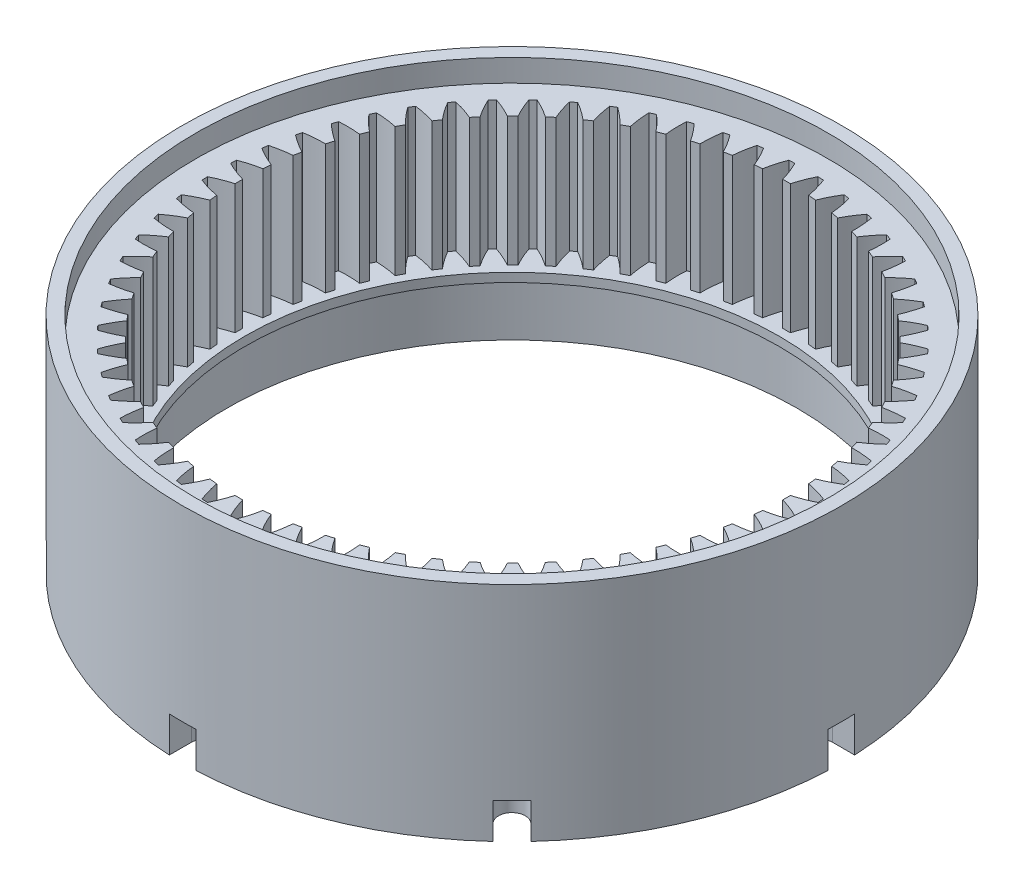
from build123d import *

# Parameters (mm, degrees)
SKETCH1_R           = 37
BOSS_EXTRUDE1_DEPTH = 25
SKETCH2_R           = 35.5
CUT_EXTRUDE1_DEPTH  = 2.5
CUT_EXTRUDE2_DEPTH  = 14.5
SKETCH4_R           = 30
CUT_EXTRUDE3_DEPTH  = 62.5
SKETCH5_R           = 32
CUT_EXTRUDE4_DEPTH  = 7
CUT_EXTRUDE5_DEPTH  = 6
CUT_EXTRUDE6_DEPTH  = 4
CIRPATTERN1_COUNT   = 8


with BuildPart() as part:
    # Sketch1 → Boss-Extrude1 (new body)
    with BuildSketch(Plane(origin=(0, 0, 0), x_dir=(1, 0, 0), z_dir=(0, 1, 0))):
        with Locations(Location((0, 0, 0), (0, 0, 270))):
            Circle(SKETCH1_R)
    extrude(amount=BOSS_EXTRUDE1_DEPTH)

    # Sketch2 → Cut-Extrude1 (cut)
    with BuildSketch(Plane(origin=(0, 25, 0), x_dir=(1, 0, 0), z_dir=(0, 1, 0))):
        with Locations(Location((0, 0, 0), (0, 0, 270))):
            Circle(SKETCH2_R)
    extrude(amount=-CUT_EXTRUDE1_DEPTH, mode=Mode.SUBTRACT)

    # Sketch3 → Cut-Extrude2 (cut)
    with BuildSketch(Plane(origin=(0, 22.5, 0), x_dir=(1, 0, 0), z_dir=(0, 1, 0))):
        with BuildLine():
            ThreePointArc((-33.098118466, 1.500835334), (-32.004134305, 1.015094225), (-30.869559771, 0.633667435))
            ThreePointArc((-30.869559771, 0.633667435), (-30.872535482, 0.205892471), (-30.869559771, -0.221882494))
            ThreePointArc((-30.869559771, -0.221882494), (-32.004134305, -0.603309284), (-33.098118466, -1.089050393))
            ThreePointArc((-33.098118466, -1.089050393), (-33.083785537, -1.413340782), (-33.066263433, -1.737474497))
            ThreePointArc((-33.066263433, -1.737474497), (-31.92993615, -2.113647431), (-30.763438539, -2.382029796))
            ThreePointArc((-30.763438539, -2.382029796), (-30.724470643, -2.808036577), (-30.679579982, -3.233460018))
            ThreePointArc((-30.679579982, -3.233460018), (-31.771304866, -3.724257885), (-32.81241024, -4.314889217))
            ThreePointArc((-32.81241024, -4.314889217), (-32.766360311, -4.636213187), (-32.717151921, -4.957068642))
            ThreePointArc((-32.717151921, -4.957068642), (-31.549424969, -5.22005065), (-30.362238291, -5.37280392))
            ThreePointArc((-30.362238291, -5.37280392), (-30.281702069, -5.792939841), (-30.19532878, -6.211914697))
            ThreePointArc((-30.19532878, -6.211914697), (-31.233690107, -6.80735699), (-32.21189028, -7.497190442))
            ThreePointArc((-32.21189028, -7.497190442), (-32.134566838, -7.812453466), (-32.054146065, -8.12694065))
            ThreePointArc((-32.054146065, -8.12694065), (-30.866265294, -8.274199071), (-29.669822805, -8.309852149))
            ThreePointArc((-29.669822805, -8.309852149), (-29.548493866, -8.72007107), (-29.42146977, -9.128562385))
            ThreePointArc((-29.42146977, -9.128562385), (-30.396467553, -9.822914668), (-31.302341922, -10.605306768))
            ThreePointArc((-31.302341922, -10.605306768), (-31.194489633, -10.911472691), (-31.083630974, -11.216562919))
            ThreePointArc((-31.083630974, -11.216562919), (-29.887036324, -11.246679574), (-28.692860421, -11.164889102))
            ThreePointArc((-28.692860421, -11.164889102), (-28.531907227, -11.561240391), (-28.365455637, -11.95531417))
            ThreePointArc((-28.365455637, -11.95531417), (-29.267700114, -12.741889452), (-30.092524615, -13.609305334))
            ThreePointArc((-30.092524615, -13.609305334), (-29.955182155, -13.903425613), (-29.814953239, -14.196180699))
            ThreePointArc((-29.814953239, -14.196180699), (-28.621168571, -14.108865548), (-27.440759819, -13.910419212))
            ThreePointArc((-27.440759819, -13.910419212), (-27.24173244, -14.28908579), (-27.037456375, -14.664946887))
            ThreePointArc((-27.037456375, -14.664946887), (-27.858258438, -15.536170017), (-28.594089559, -16.480255994))
            ThreePointArc((-28.594089559, -16.480255994), (-28.428579612, -16.759498088), (-28.260330921, -17.037098641))
            ThreePointArc((-28.260330921, -17.037098641), (-27.080853033, -16.833192577), (-25.925579414, -16.520001524))
            ThreePointArc((-25.925579414, -16.520001524), (-25.690394591, -16.877336625), (-25.450261341, -17.231365292))
            ThreePointArc((-25.450261341, -17.231365292), (-26.181716218, -18.178845916), (-26.821467503, -19.190509923))
            ThreePointArc((-26.821467503, -19.190509923), (-26.629384021, -19.452184578), (-26.434735881, -19.711957152))
            ThreePointArc((-26.434735881, -19.711957152), (-25.280923791, -19.393423903), (-24.161911222, -18.968504334))
            ThreePointArc((-24.161911222, -18.968504334), (-23.892833913, -19.301066624), (-23.619156093, -19.629853372))
            ThreePointArc((-23.619156093, -19.629853372), (-24.254219473, -20.644466733), (-24.791729768, -21.713965893))
            ThreePointArc((-24.791729768, -21.713965893), (-24.574922619, -21.955553039), (-24.355749598, -22.194995884))
            ThreePointArc((-24.355749598, -22.194995884), (-23.238715147, -21.764903097), (-22.16674033, -21.232347221))
            ThreePointArc((-22.16674033, -21.232347221), (-21.866361897, -21.536933944), (-21.561775174, -21.837312377))
            ThreePointArc((-21.561775174, -21.837312377), (-22.09433105, -22.909287194), (-22.524423837, -24.026321645))
            ThreePointArc((-22.524423837, -24.026321645), (-22.284980992, -24.245494666), (-22.043393846, -24.462301815))
            ThreePointArc((-22.043393846, -24.462301815), (-20.973894686, -23.92479152), (-19.959281325, -23.28972814))
            ThreePointArc((-19.959281325, -23.28972814), (-19.630494577, -23.56340596), (-19.297932287, -23.832483269))
            ThreePointArc((-19.297932287, -23.832483269), (-19.722851855, -24.951495838), (-20.041385105, -26.105307928))
            ThreePointArc((-20.041385105, -26.105307928), (-19.781612531, -26.299956068), (-19.519937876, -26.492039551))
            ThreePointArc((-19.519937876, -26.492039551), (-18.508273869, -25.852288265), (-17.560793245, -25.120833388))
            ThreePointArc((-17.560793245, -25.120833388), (-17.206764577, -25.360966638), (-16.849429477, -25.596151462))
            ThreePointArc((-16.849429477, -25.596151462), (-17.16262053, -26.75142508), (-17.366526593, -27.930902968))
            ThreePointArc((-17.366526593, -27.930902968), (-17.088926041, -28.09915166), (-16.809683947, -28.264661606))
            ThreePointArc((-16.809683947, -28.264661606), (-15.86559797, -27.528830485), (-14.99437484, -26.708028422))
            ThreePointArc((-14.99437484, -26.708028422), (-14.618513743, -26.912304487), (-14.239847165, -27.111331866))
            ThreePointArc((-14.239847165, -27.111331866), (-14.438293501, -28.291740618), (-14.525608651, -29.485525287))
            ThreePointArc((-14.525608651, -29.485525287), (-14.232853566, -29.625754203), (-13.938733287, -29.763096662))
            ThreePointArc((-13.938733287, -29.763096662), (-13.071317405, -28.938272161), (-12.284742123, -28.036027685))
            ThreePointArc((-12.284742123, -28.036027685), (-11.890668344, -28.202479275), (-11.494317055, -28.363432468))
            ThreePointArc((-11.494317055, -28.363432468), (-11.576107527, -29.557608371), (-11.545990872, -30.754203022))
            ThreePointArc((-11.545990872, -30.754203022), (-11.240900644, -30.865061681), (-10.93473472, -30.97291397))
            ThreePointArc((-10.93473472, -30.97291397), (-10.152342621, -30.0670396), (-9.457990338, -29.092041818))
            ThreePointArc((-9.457990338, -29.092041818), (-9.049499023, -29.219065913), (-8.639280102, -29.340394852))
            ThreePointArc((-8.639280102, -29.340394852), (-8.603627023, -30.536837341), (-8.456368602, -31.724718112))
            ThreePointArc((-8.456368602, -31.724718112), (-8.141881419, -31.805138885), (-7.826618395, -31.882462327))
            ThreePointArc((-7.826618395, -31.882462327), (-7.136784943, -30.904262155), (-6.54134265, -29.865900828))
            ThreePointArc((-6.54134265, -29.865900828), (-6.122367794, -29.952274117), (-5.702231873, -30.032810339))
            ThreePointArc((-5.702231873, -30.032810339), (-5.549478603, -31.219997017), (-5.286496595, -32.387723968))
            ThreePointArc((-5.286496595, -32.387723968), (-4.965641139, -32.436932358), (-4.64431717, -32.482982287))
            ThreePointArc((-4.64431717, -32.482982287), (-4.053685838, -31.441876913), (-3.562887971, -30.350152029))
            ThreePointArc((-3.562887971, -30.350152029), (-3.13746453, -30.39504269), (-2.711457749, -30.434010587))
            ThreePointArc((-2.711457749, -30.434010587), (-2.443075384, -31.600508197), (-2.06690245, -32.73683548))
            ThreePointArc((-2.06690245, -32.73683548), (-1.742768735, -32.754357584), (-1.418478346, -32.768690514))
            ThreePointArc((-1.418478346, -32.768690514), (-0.932737237, -31.674706353), (-0.551310447, -30.540131818))
            ThreePointArc((-0.551310447, -30.540131818), (-0.123535482, -30.543107529), (0.304239482, -30.540131818))
            ThreePointArc((0.304239482, -30.540131818), (0.685666273, -31.674706353), (1.171407382, -32.768690514))
            ThreePointArc((1.171407382, -32.768690514), (1.495697771, -32.754357584), (1.819831485, -32.73683548))
            ThreePointArc((1.819831485, -32.73683548), (2.196004419, -31.600508197), (2.464386784, -30.434010587))
            ThreePointArc((2.464386784, -30.434010587), (2.890393566, -30.39504269), (3.315817006, -30.350152029))
            ThreePointArc((3.315817006, -30.350152029), (3.806614874, -31.441876913), (4.397246205, -32.482982287))
            ThreePointArc((4.397246205, -32.482982287), (4.718570175, -32.436932358), (5.039425631, -32.387723968))
            ThreePointArc((5.039425631, -32.387723968), (5.302407638, -31.219997017), (5.455160909, -30.032810339))
            ThreePointArc((5.455160909, -30.032810339), (5.875296829, -29.952274117), (6.294271685, -29.865900828))
            ThreePointArc((6.294271685, -29.865900828), (6.889713978, -30.904262155), (7.57954743, -31.882462327))
            ThreePointArc((7.57954743, -31.882462327), (7.894810455, -31.805138885), (8.209297638, -31.724718112))
            ThreePointArc((8.209297638, -31.724718112), (8.356556059, -30.536837341), (8.392209137, -29.340394852))
            ThreePointArc((8.392209137, -29.340394852), (8.802428059, -29.219065913), (9.210919373, -29.092041818))
            ThreePointArc((9.210919373, -29.092041818), (9.905271657, -30.0670396), (10.687663756, -30.97291397))
            ThreePointArc((10.687663756, -30.97291397), (10.99382968, -30.865061681), (11.298919907, -30.754203022))
            ThreePointArc((11.298919907, -30.754203022), (11.329036562, -29.557608371), (11.24724609, -28.363432468))
            ThreePointArc((11.24724609, -28.363432468), (11.643597379, -28.202479275), (12.037671158, -28.036027685))
            ThreePointArc((12.037671158, -28.036027685), (12.82424644, -28.938272161), (13.691662323, -29.763096662))
            ThreePointArc((13.691662323, -29.763096662), (13.985782601, -29.625754203), (14.278537687, -29.485525287))
            ThreePointArc((14.278537687, -29.485525287), (14.191222536, -28.291740618), (13.992776201, -27.111331866))
            ThreePointArc((13.992776201, -27.111331866), (14.371442778, -26.912304487), (14.747303875, -26.708028422))
            ThreePointArc((14.747303875, -26.708028422), (15.618527006, -27.528830485), (16.562612982, -28.264661606))
            ThreePointArc((16.562612982, -28.264661606), (16.841855076, -28.09915166), (17.119455629, -27.930902968))
            ThreePointArc((17.119455629, -27.930902968), (16.915549565, -26.75142508), (16.602358513, -25.596151462))
            ThreePointArc((16.602358513, -25.596151462), (16.959693613, -25.360966638), (17.31372228, -25.120833388))
            ThreePointArc((17.31372228, -25.120833388), (18.261202904, -25.852288265), (19.272866911, -26.492039551))
            ThreePointArc((19.272866911, -26.492039551), (19.534541566, -26.299956068), (19.794314141, -26.105307928))
            ThreePointArc((19.794314141, -26.105307928), (19.475780891, -24.951495838), (19.050861322, -23.832483269))
            ThreePointArc((19.050861322, -23.832483269), (19.383423612, -23.56340596), (19.71221036, -23.28972814))
            ThreePointArc((19.71221036, -23.28972814), (20.726823722, -23.92479152), (21.796322881, -24.462301815))
            ThreePointArc((21.796322881, -24.462301815), (22.037910028, -24.245494666), (22.277352872, -24.026321645))
            ThreePointArc((22.277352872, -24.026321645), (21.847260086, -22.909287194), (21.314704209, -21.837312377))
            ThreePointArc((21.314704209, -21.837312377), (21.619290932, -21.536933944), (21.919669365, -21.232347221))
            ThreePointArc((21.919669365, -21.232347221), (22.991644182, -21.764903097), (24.108678633, -22.194995884))
            ThreePointArc((24.108678633, -22.194995884), (24.327851654, -21.955553039), (24.544658803, -21.713965893))
            ThreePointArc((24.544658803, -21.713965893), (24.007148509, -20.644466733), (23.372085128, -19.629853372))
            ThreePointArc((23.372085128, -19.629853372), (23.645762948, -19.301066624), (23.914840257, -18.968504334))
            ThreePointArc((23.914840257, -18.968504334), (25.033852826, -19.393423903), (26.187664916, -19.711957152))
            ThreePointArc((26.187664916, -19.711957152), (26.382313057, -19.452184578), (26.574396539, -19.190509923))
            ThreePointArc((26.574396539, -19.190509923), (25.934645254, -18.178845916), (25.203190377, -17.231365292))
            ThreePointArc((25.203190377, -17.231365292), (25.443323626, -16.877336625), (25.67850845, -16.520001524))
            ThreePointArc((25.67850845, -16.520001524), (26.833782069, -16.833192577), (28.013259956, -17.037098641))
            ThreePointArc((28.013259956, -17.037098641), (28.181508648, -16.759498088), (28.347018594, -16.480255994))
            ThreePointArc((28.347018594, -16.480255994), (27.611187473, -15.536170017), (26.79038541, -14.664946887))
            ThreePointArc((26.79038541, -14.664946887), (26.994661475, -14.28908579), (27.193688855, -13.910419212))
            ThreePointArc((27.193688855, -13.910419212), (28.374097607, -14.108865548), (29.567882275, -14.196180699))
            ThreePointArc((29.567882275, -14.196180699), (29.708111191, -13.903425613), (29.84545365, -13.609305334))
            ThreePointArc((29.84545365, -13.609305334), (29.020629149, -12.741889452), (28.118384673, -11.95531417))
            ThreePointArc((28.118384673, -11.95531417), (28.284836263, -11.561240391), (28.445789456, -11.164889102))
            ThreePointArc((28.445789456, -11.164889102), (29.63996536, -11.246679574), (30.83656001, -11.216562919))
            ThreePointArc((30.83656001, -11.216562919), (30.947418669, -10.911472691), (31.055270958, -10.605306768))
            ThreePointArc((31.055270958, -10.605306768), (30.149396589, -9.822914668), (29.174398806, -9.128562385))
            ThreePointArc((29.174398806, -9.128562385), (29.301422901, -8.72007107), (29.422751841, -8.309852149))
            ThreePointArc((29.422751841, -8.309852149), (30.619194329, -8.274199071), (31.807075101, -8.12694065))
            ThreePointArc((31.807075101, -8.12694065), (31.887495873, -7.812453466), (31.964819316, -7.497190442))
            ThreePointArc((31.964819316, -7.497190442), (30.986619143, -6.80735699), (29.948257816, -6.211914697))
            ThreePointArc((29.948257816, -6.211914697), (30.034631105, -5.792939841), (30.115167327, -5.37280392))
            ThreePointArc((30.115167327, -5.37280392), (31.302354005, -5.22005065), (32.470080956, -4.957068642))
            ThreePointArc((32.470080956, -4.957068642), (32.519289347, -4.636213187), (32.565339276, -4.314889217))
            ThreePointArc((32.565339276, -4.314889217), (31.524233902, -3.724257885), (30.432509017, -3.233460018))
            ThreePointArc((30.432509017, -3.233460018), (30.477399678, -2.808036577), (30.516367575, -2.382029796))
            ThreePointArc((30.516367575, -2.382029796), (31.682865186, -2.113647431), (32.819192468, -1.737474497))
            ThreePointArc((32.819192468, -1.737474497), (32.836714572, -1.413340782), (32.851047502, -1.089050393))
            ThreePointArc((32.851047502, -1.089050393), (31.757063341, -0.603309284), (30.622488807, -0.221882494))
            ThreePointArc((30.622488807, -0.221882494), (30.625464518, 0.205892471), (30.622488807, 0.633667435))
            ThreePointArc((30.622488807, 0.633667435), (31.757063341, 1.015094225), (32.851047502, 1.500835334))
            ThreePointArc((32.851047502, 1.500835334), (32.836714572, 1.825125723), (32.819192468, 2.149259438))
            ThreePointArc((32.819192468, 2.149259438), (31.682865186, 2.525432372), (30.516367575, 2.793814737))
            ThreePointArc((30.516367575, 2.793814737), (30.477399678, 3.219821519), (30.432509017, 3.645244959))
            ThreePointArc((30.432509017, 3.645244959), (31.524233902, 4.136042826), (32.565339276, 4.726674158))
            ThreePointArc((32.565339276, 4.726674158), (32.519289347, 5.047998128), (32.470080956, 5.368853583))
            ThreePointArc((32.470080956, 5.368853583), (31.302354005, 5.631835591), (30.115167327, 5.784588861))
            ThreePointArc((30.115167327, 5.784588861), (30.034631105, 6.204724782), (29.948257816, 6.623699638))
            ThreePointArc((29.948257816, 6.623699638), (30.986619143, 7.219141931), (31.964819316, 7.908975383))
            ThreePointArc((31.964819316, 7.908975383), (31.887495873, 8.224238407), (31.807075101, 8.538725591))
            ThreePointArc((31.807075101, 8.538725591), (30.619194329, 8.685984012), (29.422751841, 8.72163709))
            ThreePointArc((29.422751841, 8.72163709), (29.301422901, 9.131856011), (29.174398806, 9.540347326))
            ThreePointArc((29.174398806, 9.540347326), (30.149396589, 10.234699609), (31.055270958, 11.017091709))
            ThreePointArc((31.055270958, 11.017091709), (30.947418669, 11.323257632), (30.83656001, 11.62834786))
            ThreePointArc((30.83656001, 11.62834786), (29.63996536, 11.658464515), (28.445789456, 11.576674043))
            ThreePointArc((28.445789456, 11.576674043), (28.284836263, 11.973025332), (28.118384673, 12.367099111))
            ThreePointArc((28.118384673, 12.367099111), (29.020629149, 13.153674393), (29.84545365, 14.021090275))
            ThreePointArc((29.84545365, 14.021090275), (29.708111191, 14.315210554), (29.567882275, 14.60796564))
            ThreePointArc((29.567882275, 14.60796564), (28.374097607, 14.520650489), (27.193688855, 14.322204153))
            ThreePointArc((27.193688855, 14.322204153), (26.994661475, 14.700870731), (26.79038541, 15.076731828))
            ThreePointArc((26.79038541, 15.076731828), (27.611187473, 15.947954959), (28.347018594, 16.892040935))
            ThreePointArc((28.347018594, 16.892040935), (28.181508648, 17.171283029), (28.013259956, 17.448883582))
            ThreePointArc((28.013259956, 17.448883582), (26.833782069, 17.244977518), (25.67850845, 16.931786465))
            ThreePointArc((25.67850845, 16.931786465), (25.443323626, 17.289121566), (25.203190377, 17.643150233))
            ThreePointArc((25.203190377, 17.643150233), (25.934645254, 18.590630857), (26.574396539, 19.602294864))
            ThreePointArc((26.574396539, 19.602294864), (26.382313057, 19.863969519), (26.187664916, 20.123742093))
            ThreePointArc((26.187664916, 20.123742093), (25.033852826, 19.805208844), (23.914840257, 19.380289275))
            ThreePointArc((23.914840257, 19.380289275), (23.645762948, 19.712851565), (23.372085128, 20.041638313))
            ThreePointArc((23.372085128, 20.041638313), (24.007148509, 21.056251674), (24.544658803, 22.125750834))
            ThreePointArc((24.544658803, 22.125750834), (24.327851654, 22.36733798), (24.108678633, 22.606780825))
            ThreePointArc((24.108678633, 22.606780825), (22.991644182, 22.176688038), (21.919669365, 21.644132162))
            ThreePointArc((21.919669365, 21.644132162), (21.619290932, 21.948718885), (21.314704209, 22.249097318))
            ThreePointArc((21.314704209, 22.249097318), (21.847260086, 23.321072135), (22.277352872, 24.438106586))
            ThreePointArc((22.277352872, 24.438106586), (22.037910028, 24.657279607), (21.796322881, 24.874086756))
            ThreePointArc((21.796322881, 24.874086756), (20.726823722, 24.336576461), (19.71221036, 23.701513081))
            ThreePointArc((19.71221036, 23.701513081), (19.383423612, 23.975190901), (19.050861322, 24.24426821))
            ThreePointArc((19.050861322, 24.24426821), (19.475780891, 25.363280779), (19.794314141, 26.517092869))
            ThreePointArc((19.794314141, 26.517092869), (19.534541566, 26.711741009), (19.272866911, 26.903824492))
            ThreePointArc((19.272866911, 26.903824492), (18.261202904, 26.264073206), (17.31372228, 25.532618329))
            ThreePointArc((17.31372228, 25.532618329), (16.959693613, 25.772751579), (16.602358513, 26.007936403))
            ThreePointArc((16.602358513, 26.007936403), (16.915549565, 27.163210021), (17.119455629, 28.342687909))
            ThreePointArc((17.119455629, 28.342687909), (16.841855076, 28.510936601), (16.562612982, 28.676446547))
            ThreePointArc((16.562612982, 28.676446547), (15.618527006, 27.940615426), (14.747303875, 27.119813363))
            ThreePointArc((14.747303875, 27.119813363), (14.371442778, 27.324089428), (13.992776201, 27.523116807))
            ThreePointArc((13.992776201, 27.523116807), (14.191222536, 28.703525559), (14.278537687, 29.897310228))
            ThreePointArc((14.278537687, 29.897310228), (13.985782601, 30.037539144), (13.691662323, 30.174881603))
            ThreePointArc((13.691662323, 30.174881603), (12.82424644, 29.350057102), (12.037671158, 28.447812626))
            ThreePointArc((12.037671158, 28.447812626), (11.643597379, 28.614264216), (11.24724609, 28.775217409))
            ThreePointArc((11.24724609, 28.775217409), (11.329036562, 29.969393312), (11.298919907, 31.165987963))
            ThreePointArc((11.298919907, 31.165987963), (10.99382968, 31.276846622), (10.687663756, 31.384698911))
            ThreePointArc((10.687663756, 31.384698911), (9.905271657, 30.478824541), (9.210919373, 29.503826759))
            ThreePointArc((9.210919373, 29.503826759), (8.802428059, 29.630850854), (8.392209137, 29.752179794))
            ThreePointArc((8.392209137, 29.752179794), (8.356556059, 30.948622282), (8.209297638, 32.136503053))
            ThreePointArc((8.209297638, 32.136503053), (7.894810455, 32.216923826), (7.57954743, 32.294247268))
            ThreePointArc((7.57954743, 32.294247268), (6.889713978, 31.316047096), (6.294271685, 30.277685769))
            ThreePointArc((6.294271685, 30.277685769), (5.875296829, 30.364059058), (5.455160909, 30.44459528))
            ThreePointArc((5.455160909, 30.44459528), (5.302407638, 31.631781958), (5.039425631, 32.799508909))
            ThreePointArc((5.039425631, 32.799508909), (4.718570175, 32.848717299), (4.397246205, 32.894767228))
            ThreePointArc((4.397246205, 32.894767228), (3.806614874, 31.853661854), (3.315817006, 30.76193697))
            ThreePointArc((3.315817006, 30.76193697), (2.890393566, 30.806827631), (2.464386784, 30.845795528))
            ThreePointArc((2.464386784, 30.845795528), (2.196004419, 32.012293138), (1.819831485, 33.148620421))
            ThreePointArc((1.819831485, 33.148620421), (1.495697771, 33.166142525), (1.171407382, 33.180475455))
            ThreePointArc((1.171407382, 33.180475455), (0.685666273, 32.086491294), (0.304239482, 30.95191676))
            ThreePointArc((0.304239482, 30.95191676), (-0.123535482, 30.954892471), (-0.551310447, 30.95191676))
            ThreePointArc((-0.551310447, 30.95191676), (-0.932737237, 32.086491294), (-1.418478346, 33.180475455))
            ThreePointArc((-1.418478346, 33.180475455), (-1.742768735, 33.166142525), (-2.06690245, 33.148620421))
            ThreePointArc((-2.06690245, 33.148620421), (-2.443075384, 32.012293138), (-2.711457749, 30.845795528))
            ThreePointArc((-2.711457749, 30.845795528), (-3.13746453, 30.806827631), (-3.562887971, 30.76193697))
            ThreePointArc((-3.562887971, 30.76193697), (-4.053685838, 31.853661854), (-4.64431717, 32.894767228))
            ThreePointArc((-4.64431717, 32.894767228), (-4.965641139, 32.848717299), (-5.286496595, 32.799508909))
            ThreePointArc((-5.286496595, 32.799508909), (-5.549478603, 31.631781958), (-5.702231873, 30.44459528))
            ThreePointArc((-5.702231873, 30.44459528), (-6.122367794, 30.364059058), (-6.54134265, 30.277685769))
            ThreePointArc((-6.54134265, 30.277685769), (-7.136784943, 31.316047096), (-7.826618395, 32.294247268))
            ThreePointArc((-7.826618395, 32.294247268), (-8.141881419, 32.216923826), (-8.456368602, 32.136503053))
            ThreePointArc((-8.456368602, 32.136503053), (-8.603627023, 30.948622282), (-8.639280102, 29.752179794))
            ThreePointArc((-8.639280102, 29.752179794), (-9.049499023, 29.630850854), (-9.457990338, 29.503826759))
            ThreePointArc((-9.457990338, 29.503826759), (-10.152342621, 30.478824541), (-10.93473472, 31.384698911))
            ThreePointArc((-10.93473472, 31.384698911), (-11.240900644, 31.276846622), (-11.545990872, 31.165987963))
            ThreePointArc((-11.545990872, 31.165987963), (-11.576107527, 29.969393312), (-11.494317055, 28.775217409))
            ThreePointArc((-11.494317055, 28.775217409), (-11.890668344, 28.614264216), (-12.284742123, 28.447812626))
            ThreePointArc((-12.284742123, 28.447812626), (-13.071317405, 29.350057102), (-13.938733287, 30.174881603))
            ThreePointArc((-13.938733287, 30.174881603), (-14.232853566, 30.037539144), (-14.525608651, 29.897310228))
            ThreePointArc((-14.525608651, 29.897310228), (-14.438293501, 28.703525559), (-14.239847165, 27.523116807))
            ThreePointArc((-14.239847165, 27.523116807), (-14.618513743, 27.324089428), (-14.99437484, 27.119813363))
            ThreePointArc((-14.99437484, 27.119813363), (-15.86559797, 27.940615426), (-16.809683947, 28.676446547))
            ThreePointArc((-16.809683947, 28.676446547), (-17.088926041, 28.510936601), (-17.366526594, 28.342687909))
            ThreePointArc((-17.366526594, 28.342687909), (-17.16262053, 27.163210021), (-16.849429477, 26.007936403))
            ThreePointArc((-16.849429477, 26.007936403), (-17.206764577, 25.772751579), (-17.560793245, 25.532618329))
            ThreePointArc((-17.560793245, 25.532618329), (-18.508273869, 26.264073206), (-19.519937876, 26.903824492))
            ThreePointArc((-19.519937876, 26.903824492), (-19.781612531, 26.711741009), (-20.041385105, 26.517092869))
            ThreePointArc((-20.041385105, 26.517092869), (-19.722851855, 25.363280779), (-19.297932287, 24.24426821))
            ThreePointArc((-19.297932287, 24.24426821), (-19.630494577, 23.975190901), (-19.959281325, 23.701513081))
            ThreePointArc((-19.959281325, 23.701513081), (-20.973894686, 24.336576461), (-22.043393846, 24.874086756))
            ThreePointArc((-22.043393846, 24.874086756), (-22.284980992, 24.657279607), (-22.524423837, 24.438106586))
            ThreePointArc((-22.524423837, 24.438106586), (-22.09433105, 23.321072135), (-21.561775174, 22.249097318))
            ThreePointArc((-21.561775174, 22.249097318), (-21.866361897, 21.948718885), (-22.16674033, 21.644132162))
            ThreePointArc((-22.16674033, 21.644132162), (-23.238715147, 22.176688038), (-24.355749598, 22.606780825))
            ThreePointArc((-24.355749598, 22.606780825), (-24.574922619, 22.36733798), (-24.791729768, 22.125750834))
            ThreePointArc((-24.791729768, 22.125750834), (-24.254219473, 21.056251674), (-23.619156093, 20.041638313))
            ThreePointArc((-23.619156093, 20.041638313), (-23.892833913, 19.712851565), (-24.161911222, 19.380289275))
            ThreePointArc((-24.161911222, 19.380289275), (-25.280923791, 19.805208844), (-26.434735881, 20.123742093))
            ThreePointArc((-26.434735881, 20.123742093), (-26.629384021, 19.863969519), (-26.821467503, 19.602294864))
            ThreePointArc((-26.821467503, 19.602294864), (-26.181716218, 18.590630857), (-25.450261341, 17.643150233))
            ThreePointArc((-25.450261341, 17.643150233), (-25.690394591, 17.289121566), (-25.925579414, 16.931786465))
            ThreePointArc((-25.925579414, 16.931786465), (-27.080853033, 17.244977518), (-28.260330921, 17.448883582))
            ThreePointArc((-28.260330921, 17.448883582), (-28.428579612, 17.171283029), (-28.594089559, 16.892040935))
            ThreePointArc((-28.594089559, 16.892040935), (-27.858258438, 15.947954959), (-27.037456375, 15.076731828))
            ThreePointArc((-27.037456375, 15.076731828), (-27.24173244, 14.700870731), (-27.440759819, 14.322204153))
            ThreePointArc((-27.440759819, 14.322204153), (-28.621168571, 14.520650489), (-29.814953239, 14.60796564))
            ThreePointArc((-29.814953239, 14.60796564), (-29.955182155, 14.315210554), (-30.092524615, 14.021090275))
            ThreePointArc((-30.092524615, 14.021090275), (-29.267700114, 13.153674393), (-28.365455637, 12.367099111))
            ThreePointArc((-28.365455637, 12.367099111), (-28.531907227, 11.973025332), (-28.692860421, 11.576674043))
            ThreePointArc((-28.692860421, 11.576674043), (-29.887036324, 11.658464515), (-31.083630974, 11.62834786))
            ThreePointArc((-31.083630974, 11.62834786), (-31.194489633, 11.323257632), (-31.302341922, 11.017091709))
            ThreePointArc((-31.302341922, 11.017091709), (-30.396467553, 10.234699609), (-29.42146977, 9.540347326))
            ThreePointArc((-29.42146977, 9.540347326), (-29.548493866, 9.131856011), (-29.669822805, 8.72163709))
            ThreePointArc((-29.669822805, 8.72163709), (-30.866265294, 8.685984012), (-32.054146065, 8.538725591))
            ThreePointArc((-32.054146065, 8.538725591), (-32.134566838, 8.224238407), (-32.21189028, 7.908975383))
            ThreePointArc((-32.21189028, 7.908975383), (-31.233690107, 7.219141931), (-30.19532878, 6.623699638))
            ThreePointArc((-30.19532878, 6.623699638), (-30.281702069, 6.204724782), (-30.362238291, 5.784588861))
            ThreePointArc((-30.362238291, 5.784588861), (-31.549424969, 5.631835591), (-32.717151921, 5.368853583))
            ThreePointArc((-32.717151921, 5.368853583), (-32.766360311, 5.047998128), (-32.81241024, 4.726674158))
            ThreePointArc((-32.81241024, 4.726674158), (-31.771304866, 4.136042826), (-30.679579982, 3.645244959))
            ThreePointArc((-30.679579982, 3.645244959), (-30.724470643, 3.219821519), (-30.763438539, 2.793814737))
            ThreePointArc((-30.763438539, 2.793814737), (-31.92993615, 2.525432372), (-33.066263433, 2.149259438))
            ThreePointArc((-33.066263433, 2.149259438), (-33.083785537, 1.825125723), (-33.098118466, 1.500835334))
        make_face()
    extrude(amount=-CUT_EXTRUDE2_DEPTH, mode=Mode.SUBTRACT)

    # Sketch4 → Cut-Extrude3 (cut)
    with BuildSketch(Plane.XZ):
        with Locations(Location((0, 0, 0), (0, 0, 270))):
            Circle(SKETCH4_R)
    extrude(amount=-CUT_EXTRUDE3_DEPTH, mode=Mode.SUBTRACT)

    # Sketch5 → Cut-Extrude4 (cut)
    with BuildSketch(Plane.XZ):
        with Locations(Location((0, 0, 0), (0, 0, 270))):
            Circle(SKETCH5_R)
    extrude(amount=-CUT_EXTRUDE4_DEPTH, mode=Mode.SUBTRACT)

    # Sketch6 → Cut-Extrude5 (cut)
    with BuildSketch(Plane.XZ):
        with BuildLine():
            Line((22.627416998, 26.162950904), (23.626622191, 27.162156097))
            ThreePointArc((23.626622191, 27.162156097), (13.776603565, 33.25966317), (2.5, 35.913089536))
            Line((2.5, 35.913089536), (2.5, 34.5))
            ThreePointArc((2.5, 34.5), (2.359867411, 33.674757124), (1.955179357, 32.942028986))
            ThreePointArc((1.955179357, 32.942028986), (12.628553268, 30.488024573), (21.9110115, 24.676052663))
            ThreePointArc((21.9110115, 24.676052663), (22.142970869, 25.480327366), (22.627416998, 26.162950904))
        make_face()
        with BuildLine():
            Line((-2.5, 34.5), (-2.5, 35.913089536))
            ThreePointArc((-2.5, 35.913089536), (-13.776603565, 33.25966317), (-23.626622191, 27.162156097))
            Line((-23.626622191, 27.162156097), (-22.627416998, 26.162950904))
            ThreePointArc((-22.627416998, 26.162950904), (-22.142970869, 25.480327366), (-21.9110115, 24.676052663))
            ThreePointArc((-21.9110115, 24.676052663), (-12.628553268, 30.488024573), (-1.955179357, 32.942028986))
            ThreePointArc((-1.955179357, 32.942028986), (-2.359867411, 33.674757124), (-2.5, 34.5))
        make_face()
        with BuildLine():
            Line((27.162156097, 23.626622191), (26.162950904, 22.627416998))
            ThreePointArc((26.162950904, 22.627416998), (25.480327366, 22.142970869), (24.676052663, 21.9110115))
            ThreePointArc((24.676052663, 21.9110115), (30.488024573, 12.628553268), (32.942028986, 1.955179357))
            ThreePointArc((32.942028986, 1.955179357), (33.674757124, 2.359867411), (34.5, 2.5))
            Line((34.5, 2.5), (35.913089536, 2.5))
            ThreePointArc((35.913089536, 2.5), (33.25966317, 13.776603565), (27.162156097, 23.626622191))
        make_face()
        with BuildLine():
            Line((35.913089536, -2.5), (34.5, -2.5))
            ThreePointArc((34.5, -2.5), (33.674757124, -2.359867411), (32.942028986, -1.955179357))
            ThreePointArc((32.942028986, -1.955179357), (30.488024573, -12.628553268), (24.676052663, -21.9110115))
            ThreePointArc((24.676052663, -21.9110115), (25.480327366, -22.142970869), (26.162950904, -22.627416998))
            Line((26.162950904, -22.627416998), (27.162156097, -23.626622191))
            ThreePointArc((27.162156097, -23.626622191), (33.25966317, -13.776603565), (35.913089536, -2.5))
        make_face()
        with BuildLine():
            Line((23.626622191, -27.162156097), (22.627416998, -26.162950904))
            ThreePointArc((22.627416998, -26.162950904), (22.142970869, -25.480327366), (21.9110115, -24.676052663))
            ThreePointArc((21.9110115, -24.676052663), (12.628553268, -30.488024573), (1.955179357, -32.942028986))
            ThreePointArc((1.955179357, -32.942028986), (2.359867411, -33.674757124), (2.5, -34.5))
            Line((2.5, -34.5), (2.5, -35.913089536))
            ThreePointArc((2.5, -35.913089536), (13.776603565, -33.25966317), (23.626622191, -27.162156097))
        make_face()
        with BuildLine():
            Line((-2.5, -35.913089536), (-2.5, -34.5))
            ThreePointArc((-2.5, -34.5), (-2.359867411, -33.674757124), (-1.955179357, -32.942028986))
            ThreePointArc((-1.955179357, -32.942028986), (-12.628553268, -30.488024573), (-21.9110115, -24.676052663))
            ThreePointArc((-21.9110115, -24.676052663), (-22.142970869, -25.480327366), (-22.627416998, -26.162950904))
            Line((-22.627416998, -26.162950904), (-23.626622191, -27.162156097))
            ThreePointArc((-23.626622191, -27.162156097), (-13.776603565, -33.25966317), (-2.5, -35.913089536))
        make_face()
        with BuildLine():
            Line((-27.162156097, -23.626622191), (-26.162950904, -22.627416998))
            ThreePointArc((-26.162950904, -22.627416998), (-25.480327366, -22.142970869), (-24.676052663, -21.9110115))
            ThreePointArc((-24.676052663, -21.9110115), (-30.488024573, -12.628553268), (-32.942028986, -1.955179357))
            ThreePointArc((-32.942028986, -1.955179357), (-33.674757124, -2.359867411), (-34.5, -2.5))
            Line((-34.5, -2.5), (-35.913089536, -2.5))
            ThreePointArc((-35.913089536, -2.5), (-33.25966317, -13.776603565), (-27.162156097, -23.626622191))
        make_face()
        with BuildLine():
            Line((-35.913089536, 2.5), (-34.5, 2.5))
            ThreePointArc((-34.5, 2.5), (-33.674757124, 2.359867411), (-32.942028986, 1.955179357))
            ThreePointArc((-32.942028986, 1.955179357), (-30.488024573, 12.628553268), (-24.676052663, 21.9110115))
            ThreePointArc((-24.676052663, 21.9110115), (-25.480327366, 22.142970869), (-26.162950904, 22.627416998))
            Line((-26.162950904, 22.627416998), (-27.162156097, 23.626622191))
            ThreePointArc((-27.162156097, 23.626622191), (-33.25966317, 13.776603565), (-35.913089536, 2.5))
        make_face()
    extrude(amount=-CUT_EXTRUDE5_DEPTH, mode=Mode.SUBTRACT)

    # Sketch7 → Cut-Extrude6 (cut)
    with BuildSketch(Plane.XZ):
        with BuildLine():
            Line((-1.5, 34.5), (-1.5, 38.934005273))
            Line((-1.5, 38.934005273), (1.5, 38.934005273))
            Line((1.5, 38.934005273), (1.5, 34.5))
            ThreePointArc((1.5, 34.5), (0, 33), (-1.5, 34.5))
        make_face()
    cut_extrude6 = extrude(amount=-CUT_EXTRUDE6_DEPTH, mode=Mode.SUBTRACT)

    # CirPattern1: Cut-Extrude6 ×8 about axis
    cirpattern1_axis = Axis((0, 0, 0), (0, 1, 0))
    for i in range(1, CIRPATTERN1_COUNT):
        add(cut_extrude6.rotate(cirpattern1_axis, i * 360 / CIRPATTERN1_COUNT), mode=Mode.SUBTRACT)


solid = part.part
